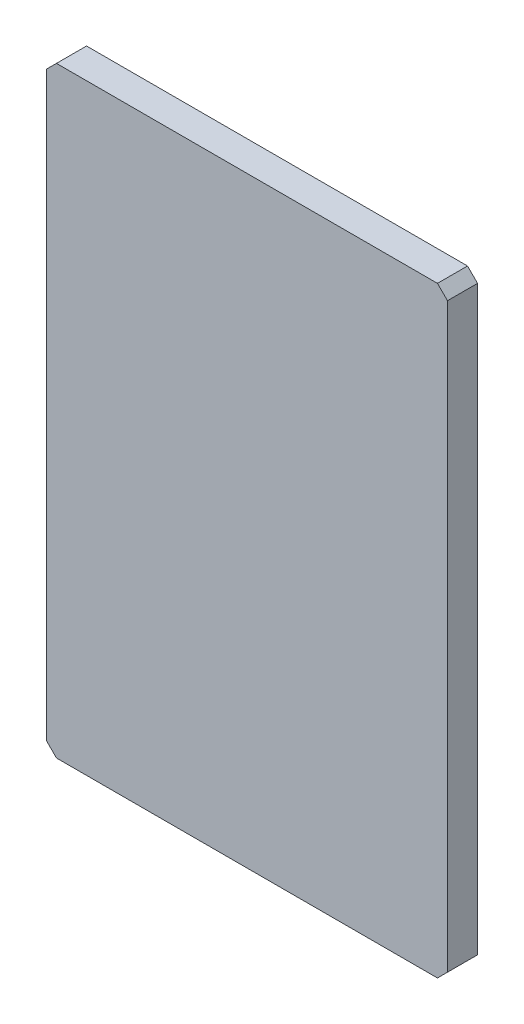
SolidWorks part; units mm, degrees
ref_plane "前视基准面" through (0, 0, 0) normal (0, 0, 1) x (1, 0, 0)
ref_plane "上视基准面" through (0, 0, 0) normal (0, 1, 0) x (1, 0, 0)
ref_plane "右视基准面" through (0, 0, 0) normal (1, 0, 0) x (0, 0, -1)
sketch "草图1" plane through (0, 0, 0) normal (0, 0, 1) x (1, 0, 0)
  line L1 (-100, -150) -> (100, -150)
  line L2 (-100, -150) -> (-100, 150)
  line L3 (-100, 150) -> (100, 150)
  line L4 (100, -150) -> (100, 150)
  line L5 (-100, -150) -> (100, 150) construction
  line L6 (-100, 150) -> (100, -150) construction
  point P0 (0, 0)
  dimension "D1" = 200
  dimension "D2" = 300
extrude "凸台-拉伸1" add sketch "草图1" along normal mid plane 15
chamfer "倒角1" distance 5 angle 45 4 edges at (-100, -150, 0) (-100, 150, 0) (100, -150, 0) (100, 150, 0)
